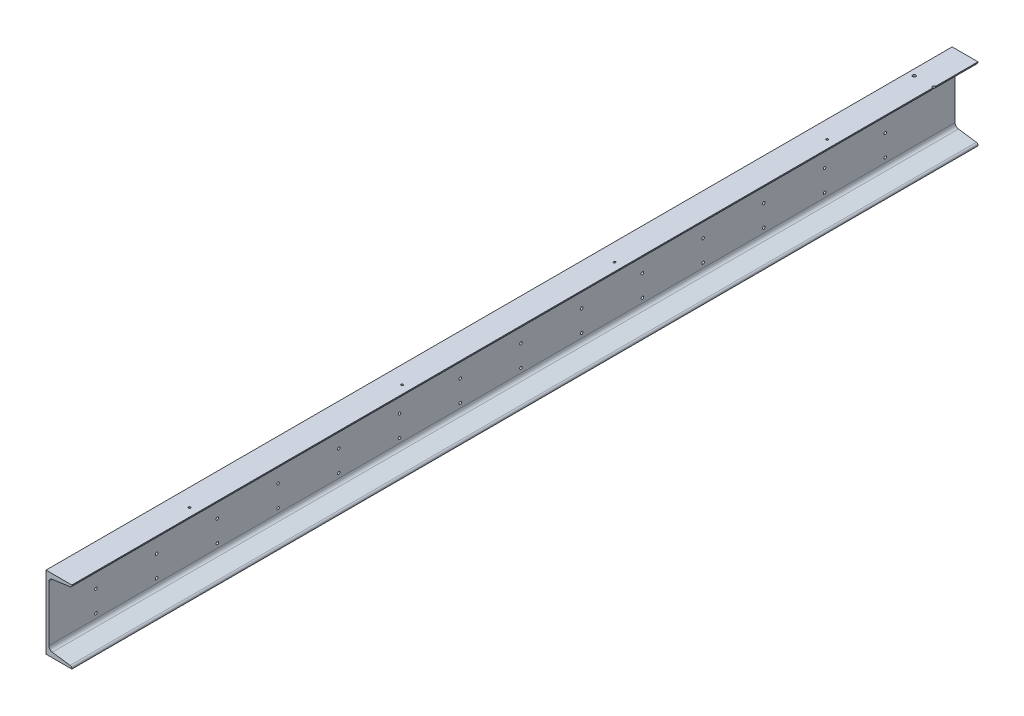
from build123d import *

# Parameters (mm, degrees)
EXTRUDE_1_DEPTH         = 2985
HOLE_WIZARD_M10_2_D     = 8.5
HOLE_WIZARD_M10_2_DEPTH = 24.5
HOLE_WIZARD_M10_2_TIP   = 2.553657631
HOLE_WIZARD_M8_1_D      = 6.8
HOLE_WIZARD_M8_1_DEPTH  = 19.75
HOLE_WIZARD_M8_1_TIP    = 2.042926105
HOLE_WIZARD_M12_1_D     = 10.2
HOLE_WIZARD_M12_1_DEPTH = 29.25
HOLE_WIZARD_M12_1_TIP   = 3.064389157
SKETCH_13_R             = 22.5
CUT_EXTRUDE_1_DEPTH     = 10
HOLE_WIZARD_M6_1_D      = 5
HOLE_WIZARD_M6_1_DEPTH  = 15
HOLE_WIZARD_M6_1_TIP    = 1.502151548


with BuildPart() as part:
    # 草图1 → 凸台-拉伸1 (new body)
    with BuildSketch(Plane.XY):
        with BuildLine():
            Line((0, 0), (-85, 0))
            Line((-85, 0), (-85, -240))
            Line((-85, -240), (0, -240))
            Line((0, -240), (0, -238.623349271))
            ThreePointArc((0, -238.623349271), (-1.594387729, -234.358965582), (-5.595374844, -232.186606824))
            Line((-5.595374844, -232.186606824), (-64.309250312, -223.934909757))
            ThreePointArc((-64.309250312, -223.934909757), (-72.311224543, -219.59019224), (-75.5, -211.061424863))
            Line((-75.5, -211.061424863), (-75.5, -28.938575137))
            ThreePointArc((-75.5, -28.938575137), (-72.311224543, -20.40980776), (-64.309250312, -16.065090243))
            Line((-64.309250312, -16.065090243), (-5.595374844, -7.813393176))
            ThreePointArc((-5.595374844, -7.813393176), (-1.594387729, -5.641034418), (0, -1.376650729))
            Line((0, -1.376650729), (0, 0))
        make_face()
    extrude(amount=EXTRUDE_1_DEPTH)

    # M10 螺纹孔2
    with Locations(Plane.ZY.offset(85)):
        with Locations((230, -126), (230, -196), (430, -126), (430, -196), (630, -126), (630, -196), (830, -126), (830, -196), (1030, -126), (1030, -196), (1230, -126), (1230, -196), (1430, -126), (1430, -196), (1630, -196), (1630, -126), (1830, -196), (1830, -126), (2030, -126), (2030, -196), (2230, -196), (2230, -126), (2430, -126), (2430, -196), (2630, -196), (2630, -126), (2830, -126), (2830, -196)):
            Hole(HOLE_WIZARD_M10_2_D / 2, depth=HOLE_WIZARD_M10_2_DEPTH)
            with Locations((0, 0, -(HOLE_WIZARD_M10_2_DEPTH + HOLE_WIZARD_M10_2_TIP / 2))):  # 118° drill point
                Cone(0, HOLE_WIZARD_M10_2_D / 2, HOLE_WIZARD_M10_2_TIP, mode=Mode.SUBTRACT)

    # M8 螺纹孔1
    with Locations(Plane(origin=(0, 0, 0), x_dir=(1, 0, 0), z_dir=(0, 1, 0))):
        with Locations((-27, -470), (-27, -1170), (-27, -1870), (-27, -2570)):
            Hole(HOLE_WIZARD_M8_1_D / 2, depth=HOLE_WIZARD_M8_1_DEPTH)
            with Locations((0, 0, -(HOLE_WIZARD_M8_1_DEPTH + HOLE_WIZARD_M8_1_TIP / 2))):  # 118° drill point
                Cone(0, HOLE_WIZARD_M8_1_D / 2, HOLE_WIZARD_M8_1_TIP, mode=Mode.SUBTRACT)

    # M12 螺纹孔1
    with Locations(Plane(origin=(0, 0, 0), x_dir=(1, 0, 0), z_dir=(0, 1, 0))):
        with Locations((-65, -145), (0, -145)):
            Hole(HOLE_WIZARD_M12_1_D / 2, depth=HOLE_WIZARD_M12_1_DEPTH)
            with Locations((0, 0, -(HOLE_WIZARD_M12_1_DEPTH + HOLE_WIZARD_M12_1_TIP / 2))):  # 118° drill point
                Cone(0, HOLE_WIZARD_M12_1_D / 2, HOLE_WIZARD_M12_1_TIP, mode=Mode.SUBTRACT)

    # 草图13 → 切除-拉伸1 (cut)
    with BuildSketch(Plane.ZY.offset(85)):
        with Locations(Location((1385, -50, 0), (0, 0, 270))):
            Circle(SKETCH_13_R)
    extrude(amount=-CUT_EXTRUDE_1_DEPTH, mode=Mode.SUBTRACT)

    # M6 螺纹孔1
    with Locations(Plane.ZY.offset(85)):
        with Locations((1675, -50), (2785, -50)):
            Hole(HOLE_WIZARD_M6_1_D / 2, depth=HOLE_WIZARD_M6_1_DEPTH)
            with Locations((0, 0, -(HOLE_WIZARD_M6_1_DEPTH + HOLE_WIZARD_M6_1_TIP / 2))):  # 118° drill point
                Cone(0, HOLE_WIZARD_M6_1_D / 2, HOLE_WIZARD_M6_1_TIP, mode=Mode.SUBTRACT)


solid = part.part
